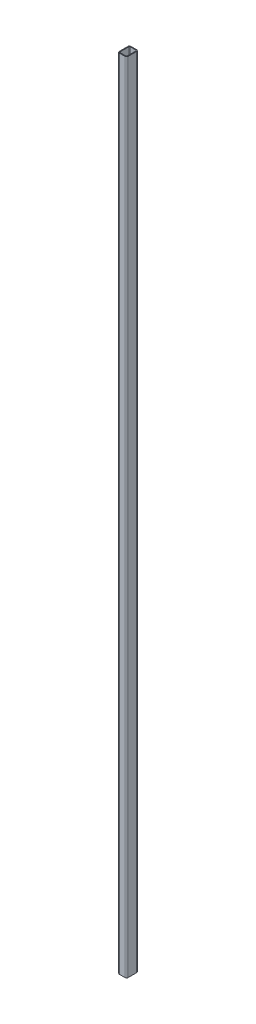
from build123d import *

# Parameters (mm, degrees)
COLD_FORMED_HOLLOW_STRUCTURAL_RECTANGULA_DEPTH = 5500


with BuildPart() as part:
    # Sketch1 → Cold-formed Hollow Structural Rectangular Steel(gb t6728-2002) 80×60×5(1) (new body)
    with BuildSketch(Plane(origin=(0, 0, 0), x_dir=(-1, 0, 0), z_dir=(0, 1, 0))):
        with BuildLine():
            Line((-20, -40), (20, -40))
            ThreePointArc((20, -40), (27.071067812, -37.071067812), (30, -30))
            Line((30, -30), (30, 30))
            ThreePointArc((30, 30), (27.071067812, 37.071067812), (20, 40))
            Line((20, 40), (-20, 40))
            ThreePointArc((-20, 40), (-27.071067812, 37.071067812), (-30, 30))
            Line((-30, 30), (-30, -30))
            ThreePointArc((-30, -30), (-27.071067812, -37.071067812), (-20, -40))
        make_face()
        with BuildLine():
            Line((-20, -35), (20, -35))
            ThreePointArc((20, -35), (23.535533906, -33.535533906), (25, -30))
            Line((25, -30), (25, 30))
            ThreePointArc((25, 30), (23.535533906, 33.535533906), (20, 35))
            Line((20, 35), (-20, 35))
            ThreePointArc((-20, 35), (-23.535533906, 33.535533906), (-25, 30))
            Line((-25, 30), (-25, -30))
            ThreePointArc((-25, -30), (-23.535533906, -33.535533906), (-20, -35))
        make_face(mode=Mode.SUBTRACT)
    extrude(amount=COLD_FORMED_HOLLOW_STRUCTURAL_RECTANGULA_DEPTH)


solid = part.part
